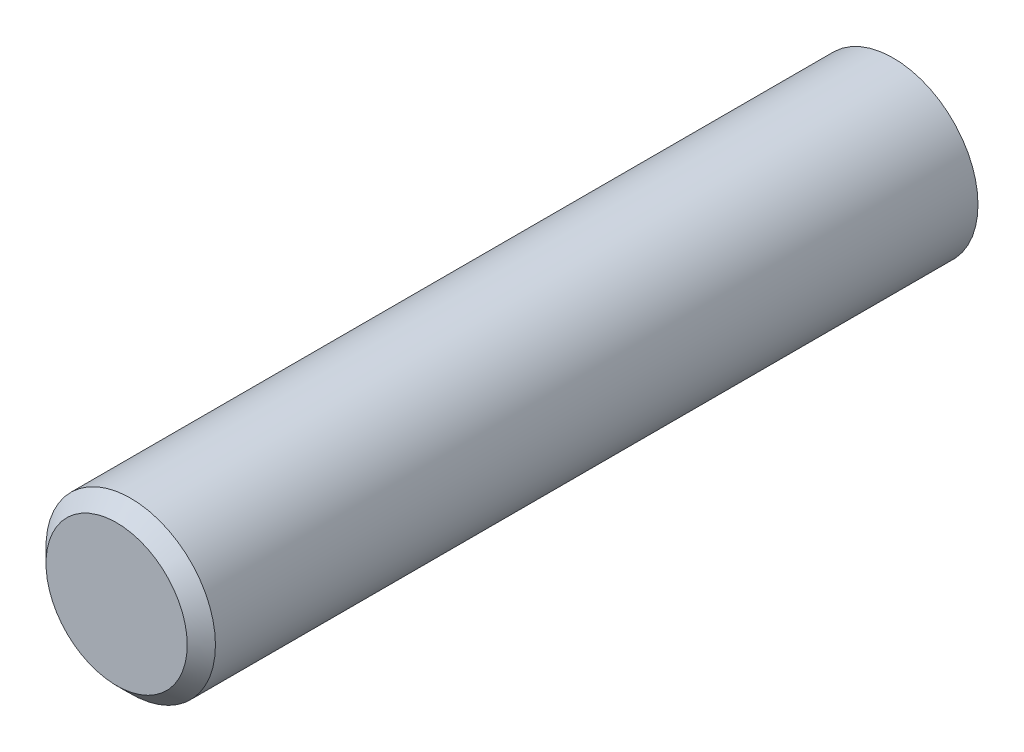
SolidWorks part; units mm, degrees
ref_plane "Front Plane" through (0, 0, 0) normal (0, 0, 1) x (1, 0, 0)
ref_plane "Top Plane" through (0, 0, 0) normal (0, 1, 0) x (1, 0, 0)
ref_plane "Right Plane" through (0, 0, 0) normal (1, 0, 0) x (0, 0, -1)
sketch "Sketch1" plane through (0, 0, 0) normal (0, 0, 1) x (1, 0, 0)
  circle A0 centre (0, 0) radius 6
extrude "Boss-Extrude1" add sketch "Sketch1" along normal blind 55
cosmetic thread "Cosmetic Thread1" parameters "D2"=10.106
chamfer "Chamfer1" distance 1 angle 45 1 edges at (6, 0, 55)
sketch "Sketch2" plane through (0, 0, 55) normal (0, 0, 1) x (1, 0, 0)
  circle A0 centre (0, 0) radius 6
